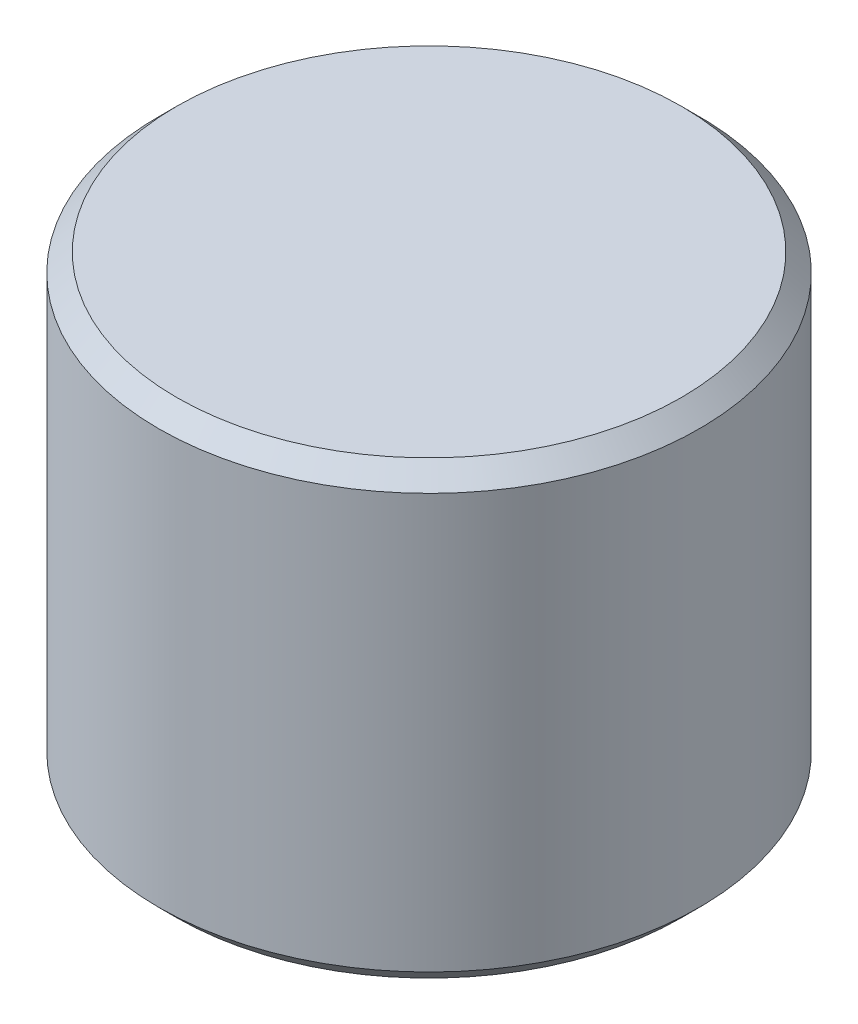
SolidWorks part; units mm, degrees
ref_plane "Front Plane" through (0, 0, 0) normal (0, 0, 1) x (1, 0, 0)
ref_plane "Top Plane" through (0, 0, 0) normal (0, 1, 0) x (1, 0, 0)
ref_plane "Right Plane" through (0, 0, 0) normal (1, 0, 0) x (0, 0, -1)
sketch "Sketch1" plane through (0, 0, 0) normal (0, 1, 0) x (1, 0, 0)
  circle A0 centre (0, 0) radius 3
  dimension "D1" = 6
extrude "Boss-Extrude1" add sketch "Sketch1" along normal blind 5
chamfer "Chamfer1" distance 0.2 angle 45 2 edges at (0, 0, 3) (0, 5, 3)
